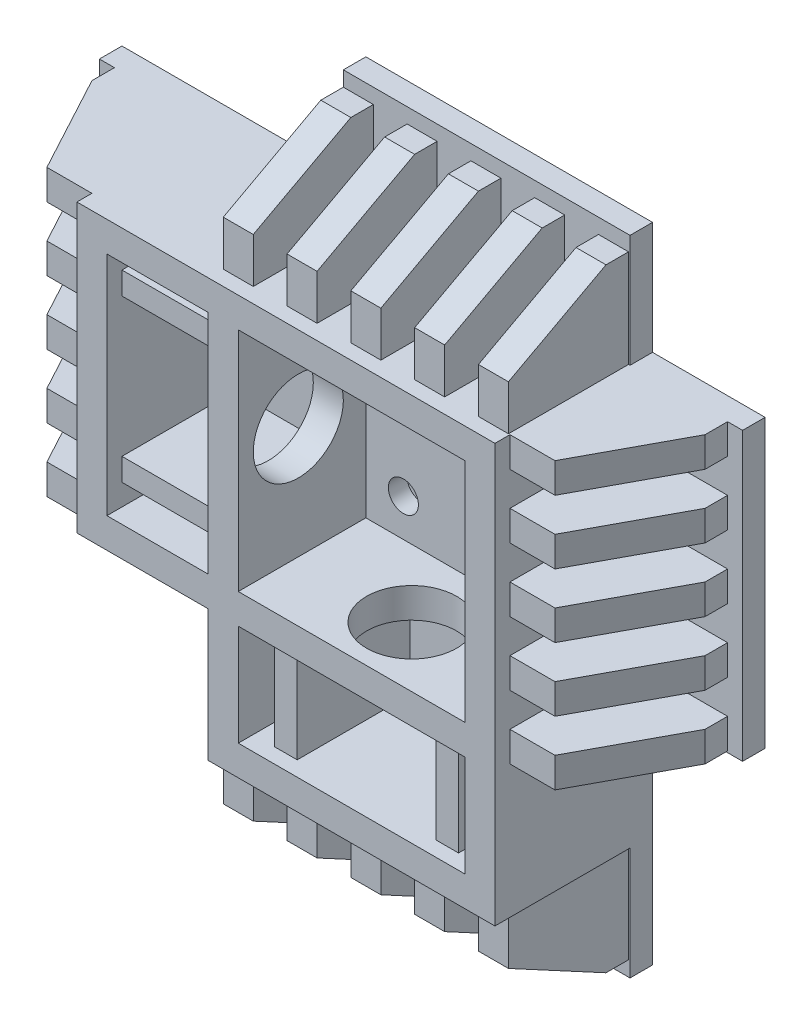
from build123d import *

# Parameters (mm, degrees)
BOSS_EXTRUDE1_DEPTH = 30
BOSS_EXTRUDE2_DEPTH = 210
SKETCH6_W           = 302
SKETCH6_H           = 302
SKETCH6_W_2         = 135
SKETCH6_H_2         = 135
CUT_EXTRUDE3_DEPTH  = 170
SKETCH7_R           = 60
CUT_EXTRUDE4_DEPTH  = 148
SKETCH8_W           = 130
SKETCH8_H           = 40
BOSS_EXTRUDE3_DEPTH = 160
SKETCH9_W           = 40
SKETCH9_H           = 130
BOSS_EXTRUDE4_DEPTH = 160
SKETCH10_W          = 135
SKETCH10_H          = 30
SKETCH10_W_2        = 30
SKETCH10_H_2        = 135
BOSS_EXTRUDE5_DEPTH = 150
CUT_EXTRUDE5_DEPTH  = 663
CUT_EXTRUDE6_DEPTH  = 663
SKETCH14_R          = 60
CUT_EXTRUDE7_DEPTH  = 60
SKETCH16_R          = 13
CUT_EXTRUDE10_DEPTH = 40
SKETCH18_R          = 20
CUT_EXTRUDE11_DEPTH = 25


with BuildPart() as part:
    # Sketch1 → Boss-Extrude1 (new body)
    with BuildSketch(Plane.XY):
        Polygon((278.5, -428.5), (278.5, -103.5), (428.5, -103.5), (428.5, 278.5), (278.5, 278.5), (278.5, 428.5), (-103.5, 428.5), (-103.5, 278.5), (-428.5, 278.5), (-428.5, -103.5), (-103.5, -103.5), (-103.5, -428.5), align=None)
    extrude(amount=BOSS_EXTRUDE1_DEPTH)

    # Sketch4 → Boss-Extrude2 (add)
    with BuildSketch(Plane(origin=(0, 0, 0), x_dir=(-1, 0, 0), z_dir=(0, 0, -1))):
        Polygon((-278.5, -278.5), (103.5, -278.5), (103.5, -103.5), (278.5, -103.5), (278.5, 278.5), (103.5, 278.5), (-278.5, 278.5), align=None)
    extrude(amount=-BOSS_EXTRUDE2_DEPTH)

    # Sketch6 → Cut-Extrude3 (cut)
    with BuildSketch(Plane.XY.offset(210)):
        with Locations((87.5, 87.5)):
            Rectangle(SKETCH6_W, SKETCH6_H)
        with Locations((-171, 87.5)):
            Rectangle(SKETCH6_W_2, SKETCH6_H)
        with Locations((87.5, -171)):
            Rectangle(SKETCH6_W, SKETCH6_H_2)
    extrude(amount=-CUT_EXTRUDE3_DEPTH, mode=Mode.SUBTRACT)

    # Sketch7 → Cut-Extrude4 (cut)
    with BuildSketch(Plane(origin=(-63.5, 0, 0), x_dir=(0, 0, -1), z_dir=(1, 0, 0))):
        with Locations(Location((-130, 87.5, 0), (0, 0, 90))):
            Circle(SKETCH7_R)
    extrude(amount=-CUT_EXTRUDE4_DEPTH, mode=Mode.SUBTRACT)

    # Sketch8 → Boss-Extrude3 (add)
    with BuildSketch(Plane.XY.offset(30)):
        with Locations((-343.5, 258.5)):
            Rectangle(SKETCH8_W, SKETCH8_H)
        with Locations((-343.5, 173.5)):
            Rectangle(SKETCH8_W, SKETCH8_H)
        with Locations((-343.5, 88.5)):
            Rectangle(SKETCH8_W, SKETCH8_H)
        with Locations((-343.5, 3.5)):
            Rectangle(SKETCH8_W, SKETCH8_H)
        with Locations((-343.5, -81.5)):
            Rectangle(SKETCH8_W, SKETCH8_H)
        with Locations((343.5, 173.5)):
            Rectangle(SKETCH8_W, SKETCH8_H)
        with Locations((343.5, 258.5)):
            Rectangle(SKETCH8_W, SKETCH8_H)
        with Locations((343.5, 88.5)):
            Rectangle(SKETCH8_W, SKETCH8_H)
        with Locations((343.5, 3.5)):
            Rectangle(SKETCH8_W, SKETCH8_H)
        with Locations((343.5, -81.5)):
            Rectangle(SKETCH8_W, SKETCH8_H)
    extrude(amount=BOSS_EXTRUDE3_DEPTH)

    # Sketch9 → Boss-Extrude4 (add)
    with BuildSketch(Plane.XY.offset(30)):
        with Locations((1.5, -343.5)):
            Rectangle(SKETCH9_W, SKETCH9_H)
        with Locations((-83.5, -343.5)):
            Rectangle(SKETCH9_W, SKETCH9_H)
        with Locations((-83.5, 343.5)):
            Rectangle(SKETCH9_W, SKETCH9_H)
        with Locations((1.5, 343.5)):
            Rectangle(SKETCH9_W, SKETCH9_H)
        with Locations((86.5, -343.5)):
            Rectangle(SKETCH9_W, SKETCH9_H)
        with Locations((86.5, 343.5)):
            Rectangle(SKETCH9_W, SKETCH9_H)
        with Locations((171.5, -343.5)):
            Rectangle(SKETCH9_W, SKETCH9_H)
        with Locations((171.5, 343.5)):
            Rectangle(SKETCH9_W, SKETCH9_H)
        with Locations((256.5, -343.5)):
            Rectangle(SKETCH9_W, SKETCH9_H)
        with Locations((256.5, 343.5)):
            Rectangle(SKETCH9_W, SKETCH9_H)
    extrude(amount=BOSS_EXTRUDE4_DEPTH)

    # Sketch10 → Boss-Extrude5 (add)
    with BuildSketch(Plane.XY.offset(40)):
        with Locations((-171, 195)):
            Rectangle(SKETCH10_W, SKETCH10_H)
        with Locations((-171, -20)):
            Rectangle(SKETCH10_W, SKETCH10_H)
        with Locations((-20, -171)):
            Rectangle(SKETCH10_W_2, SKETCH10_H_2)
        with Locations((195, -171)):
            Rectangle(SKETCH10_W_2, SKETCH10_H_2)
    extrude(amount=BOSS_EXTRUDE5_DEPTH)

    # Sketch11 → Cut-Extrude5 (cut)
    with BuildSketch(Plane.XZ.offset(101.5)):
        Polygon((-338.5, 190), (-408.5, 60), (-408.5, 190), align=None)
        Polygon((338.5, 190), (408.5, 60), (408.5, 190), align=None)
    extrude(amount=-CUT_EXTRUDE5_DEPTH, mode=Mode.SUBTRACT)

    # Sketch12 → Cut-Extrude6 (cut)
    with BuildSketch(Plane(origin=(276.5, 0, 0), x_dir=(0, 0, -1), z_dir=(1, 0, 0))):
        Polygon((-60, 408.5), (-190, 338.5), (-190, 408.5), align=None)
        Polygon((-190, -338.5), (-60, -408.5), (-190, -408.5), align=None)
    extrude(amount=-CUT_EXTRUDE6_DEPTH, mode=Mode.SUBTRACT)

    # Sketch14 → Cut-Extrude7 (cut)
    with BuildSketch(Plane(origin=(0, -63.5, 0), x_dir=(1, 0, 0), z_dir=(0, 1, 0))):
        with Locations(Location((87.5, -130, 0), (0, 0, 180))):
            Circle(SKETCH14_R)
    extrude(amount=-CUT_EXTRUDE7_DEPTH, mode=Mode.SUBTRACT)

    # Sketch16 → Cut-Extrude10 (cut)
    with BuildSketch(Plane.XY.offset(40)):
        with Locations((-13.5, 188.5)):
            Circle(SKETCH16_R)
        with Locations((188.5, 188.5)):
            Circle(SKETCH16_R)
        with Locations((-13.5, -13.5)):
            Circle(SKETCH16_R)
        with Locations((188.5, -13.5)):
            Circle(SKETCH16_R)
    extrude(amount=-CUT_EXTRUDE10_DEPTH, mode=Mode.SUBTRACT)

    # Sketch18 → Cut-Extrude11 (cut)
    with BuildSketch(Plane.XY.offset(40)):
        with Locations((-13.5, 188.5)):
            Circle(SKETCH18_R)
        with Locations((188.5, 188.5)):
            Circle(SKETCH18_R)
        with Locations((-13.5, -13.5)):
            Circle(SKETCH18_R)
        with Locations((188.5, -13.5)):
            Circle(SKETCH18_R)
    extrude(amount=-CUT_EXTRUDE11_DEPTH, mode=Mode.SUBTRACT)


solid = part.part
